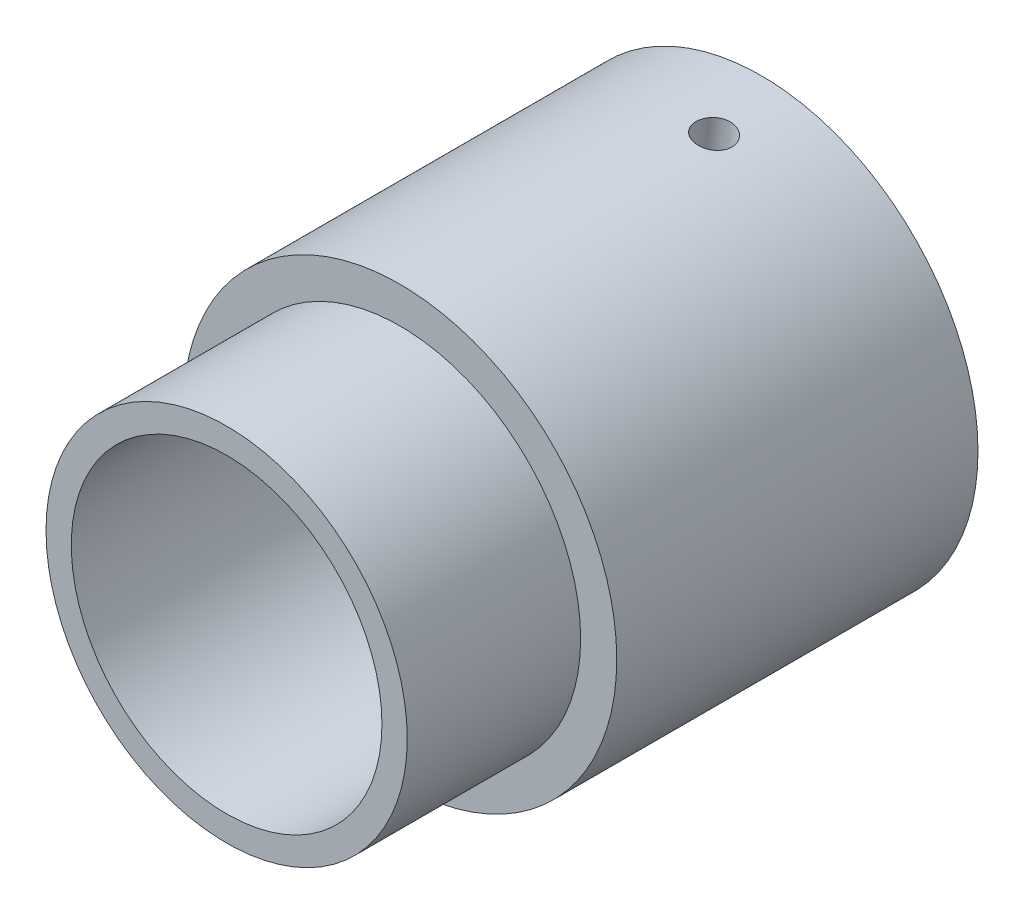
from build123d import *

# Parameters (mm, degrees)
SKETCH1_R             = 30
SKETCH1_R_2           = 21.5
BOSS_EXTRUDE1_DEPTH   = 50
M6_TAPPED_HOLE1_D     = 5
M6_TAPPED_HOLE1_DEPTH = 18
M6_TAPPED_HOLE1_TIP   = 1.502151548
BOSS_EXTRUDE2_START   = 24
SKETCH4_R             = 25
SKETCH4_R_2           = 21.5
BOSS_EXTRUDE2_DEPTH   = 24


with BuildPart() as part:
    # Sketch1 → Boss-Extrude1 (new body)
    with BuildSketch(Plane.XY):
        Circle(SKETCH1_R)
        Circle(SKETCH1_R_2, mode=Mode.SUBTRACT)
    extrude(amount=-BOSS_EXTRUDE1_DEPTH)

    # M6 Tapped Hole1
    with Locations(Plane(origin=(3.471069712, 29.798518001, -40), x_dir=(0.993283933364, -0.115702323745, 0), z_dir=(0.115702323745, 0.993283933364, 0))):
        with Locations((0, 0)):
            Hole(M6_TAPPED_HOLE1_D / 2, depth=M6_TAPPED_HOLE1_DEPTH)
            with Locations((0, 0, -(M6_TAPPED_HOLE1_DEPTH + M6_TAPPED_HOLE1_TIP / 2))):  # 118° drill point
                Cone(0, M6_TAPPED_HOLE1_D / 2, M6_TAPPED_HOLE1_TIP, mode=Mode.SUBTRACT)

    # Sketch4 → Boss-Extrude2 (add)
    with BuildSketch(Plane.XY.offset(BOSS_EXTRUDE2_START)):
        Circle(SKETCH4_R)
        Circle(SKETCH4_R_2, mode=Mode.SUBTRACT)
    extrude(amount=-BOSS_EXTRUDE2_DEPTH)


solid = part.part
